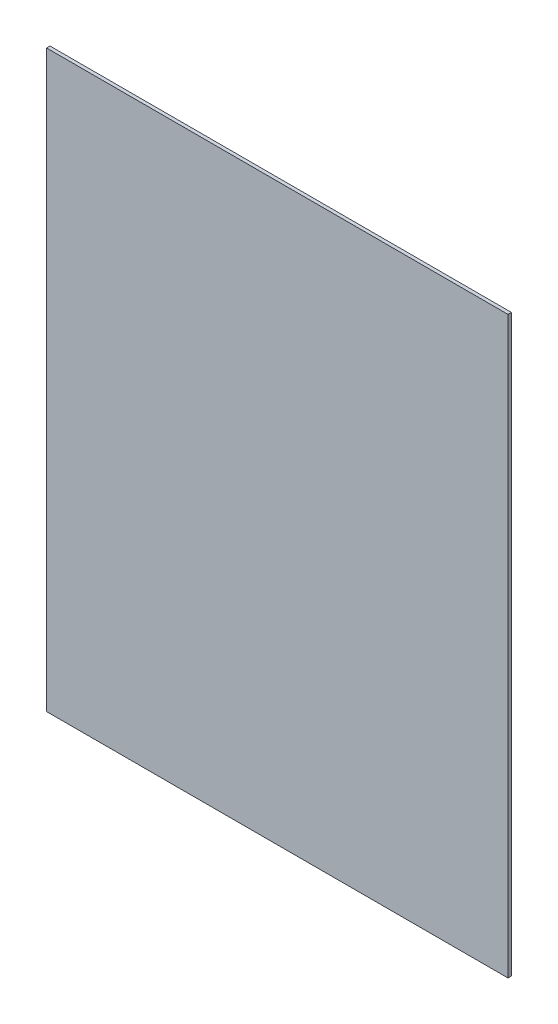
from build123d import *

# Parameters (mm, degrees)
SKETCH_1_W      = 676
SKETCH_1_H      = 842
EXTRUDE_1_DEPTH = 5


with BuildPart() as part:
    # 草图1 → 凸台-拉伸1 (new body)
    with BuildSketch(Plane.XY):
        Rectangle(SKETCH_1_W, SKETCH_1_H)
    extrude(amount=EXTRUDE_1_DEPTH)


solid = part.part
